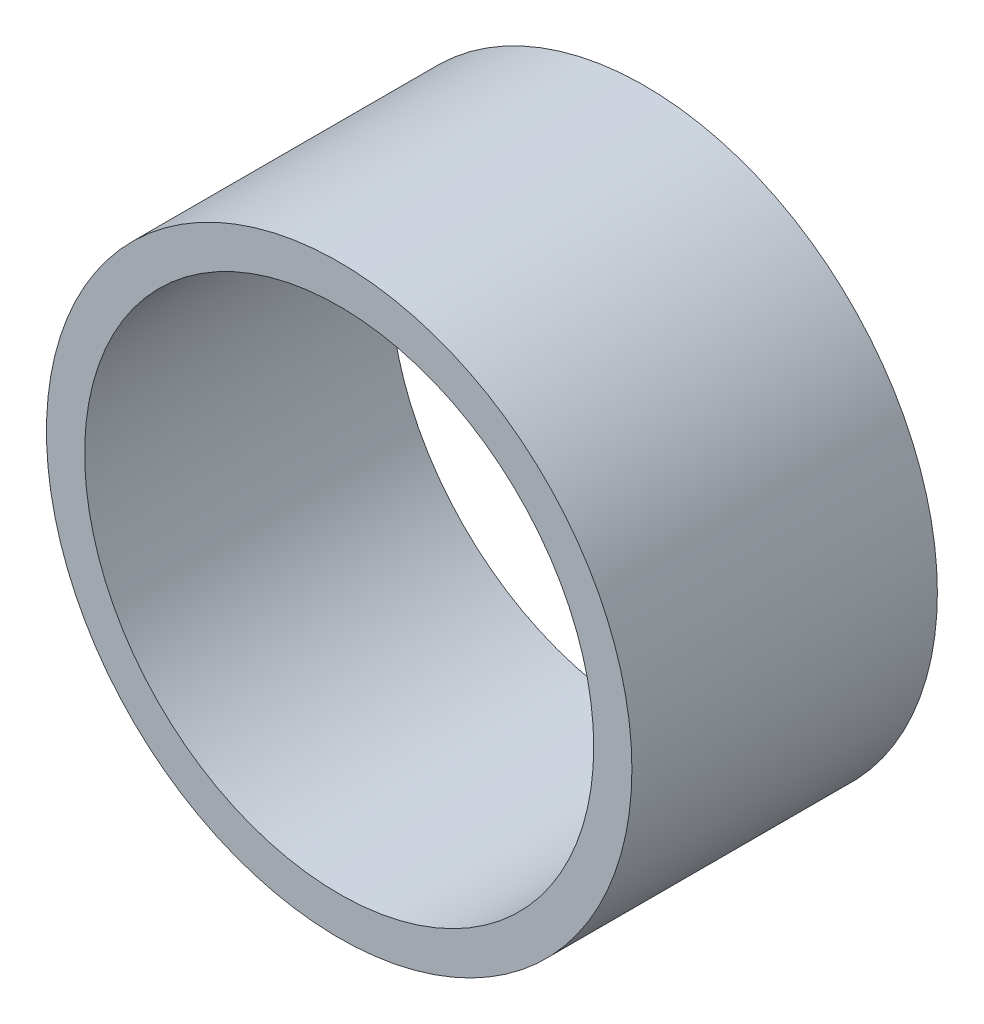
from build123d import *

# Parameters (mm, degrees)
SKETCH1_R           = 11.5
SKETCH1_R_2         = 10
BOSS_EXTRUDE1_DEPTH = 12


with BuildPart() as part:
    # Sketch1 → Boss-Extrude1 (new body)
    with BuildSketch(Plane.XY):
        Circle(SKETCH1_R)
        Circle(SKETCH1_R_2, mode=Mode.SUBTRACT)
    extrude(amount=BOSS_EXTRUDE1_DEPTH)


solid = part.part
